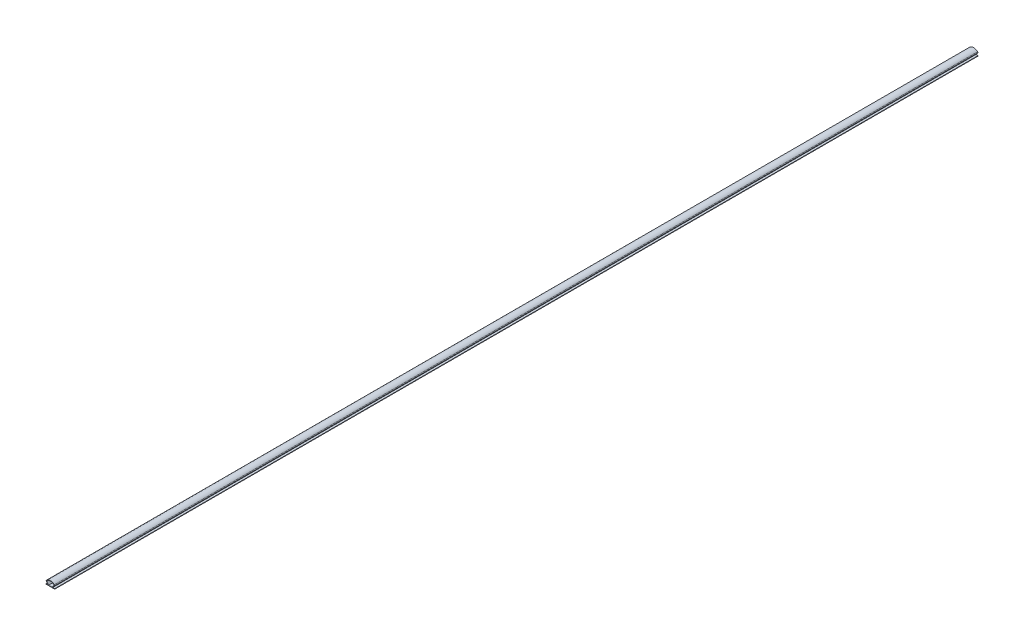
from build123d import *

# Parameters (mm, degrees)
EXTRUDE_1_DEPTH = 529


with BuildPart() as part:
    # 草图1 → 凸台-拉伸1 (new, symmetric)
    with BuildSketch(Plane.XY):
        with BuildLine():
            Line((-4.556913863, 4.138102128), (-2.645672962, 1.79891143))
            Line((-2.645672962, 1.79891143), (-5, 1.79891143))
            Line((-5, 1.79891143), (-5, 1.29891143))
            Line((-5, 1.29891143), (1.591473901, 1.29891143))
            Line((1.591473901, 1.29891143), (5, 1.29891143))
            Line((5, 1.29891143), (5, 1.79891143))
            Line((5, 1.79891143), (2.645672962, 1.79891143))
            Line((2.645672962, 1.79891143), (4.556913863, 4.138102128))
            ThreePointArc((4.556913863, 4.138102128), (4.780792009, 4.829714088), (4.47713902, 5.490201325))
            ThreePointArc((4.47713902, 5.490201325), (0, 7.29891143), (-4.47713902, 5.490201325))
            ThreePointArc((-4.47713902, 5.490201325), (-4.780792009, 4.829714088), (-4.556913863, 4.138102128))
        make_face()
        with BuildLine():
            Line((-2, 1.79891143), (2, 1.79891143))
            Line((2, 1.79891143), (4.169720942, 4.454458955))
            ThreePointArc((4.169720942, 4.454458955), (4.281660015, 4.800264935), (4.12983352, 5.130508554))
            ThreePointArc((4.12983352, 5.130508554), (0, 6.79891143), (-4.12983352, 5.130508554))
            ThreePointArc((-4.12983352, 5.130508554), (-4.281660015, 4.800264935), (-4.169720942, 4.454458955))
            Line((-4.169720942, 4.454458955), (-2, 1.79891143))
        make_face(mode=Mode.SUBTRACT)
    extrude(amount=EXTRUDE_1_DEPTH, both=True)


solid = part.part
